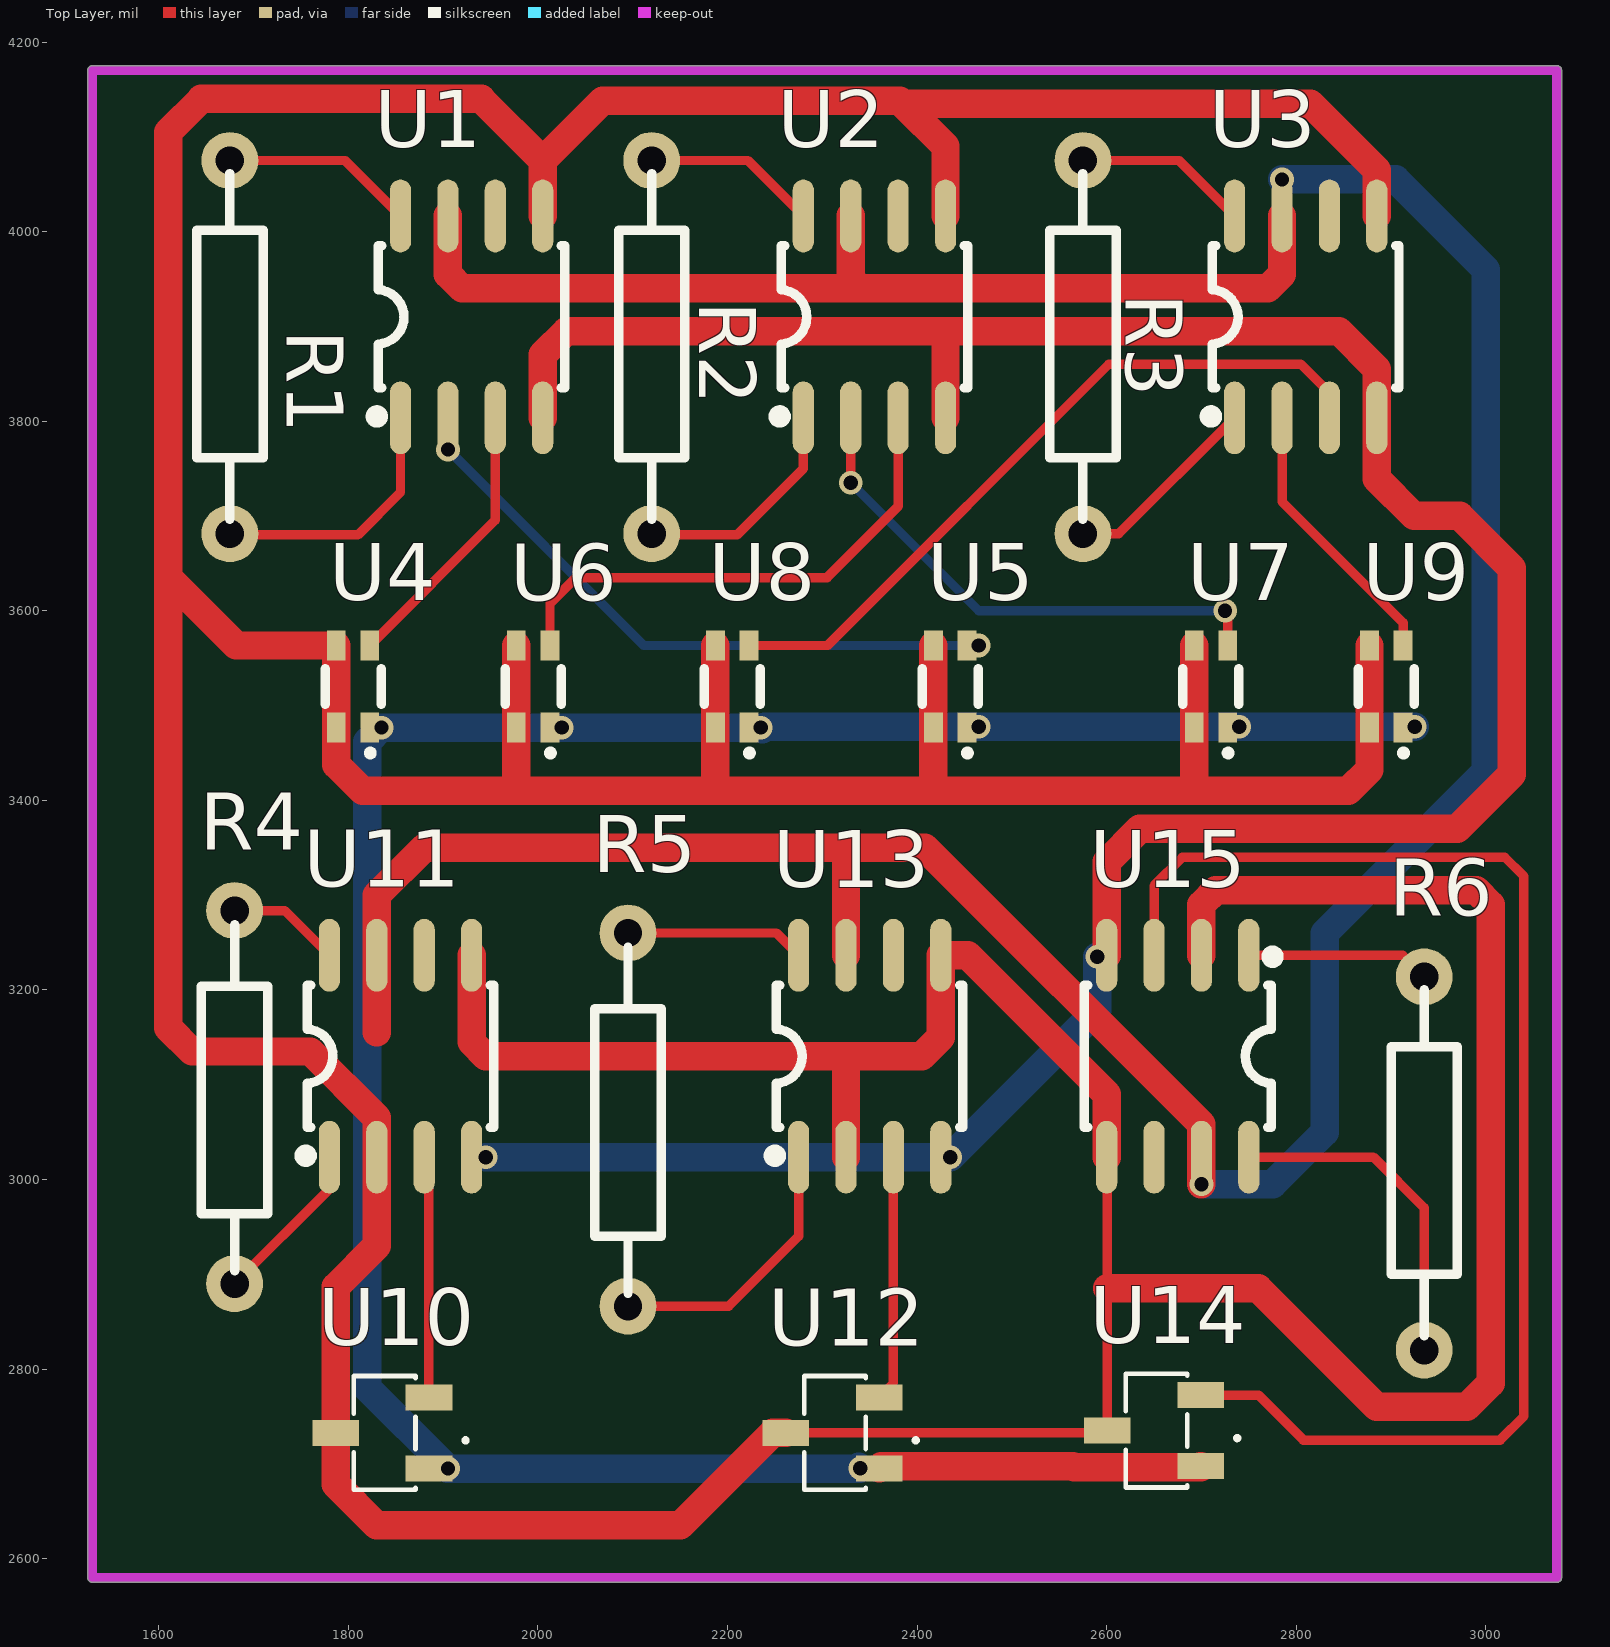
[diagram p0: Top Layer view]
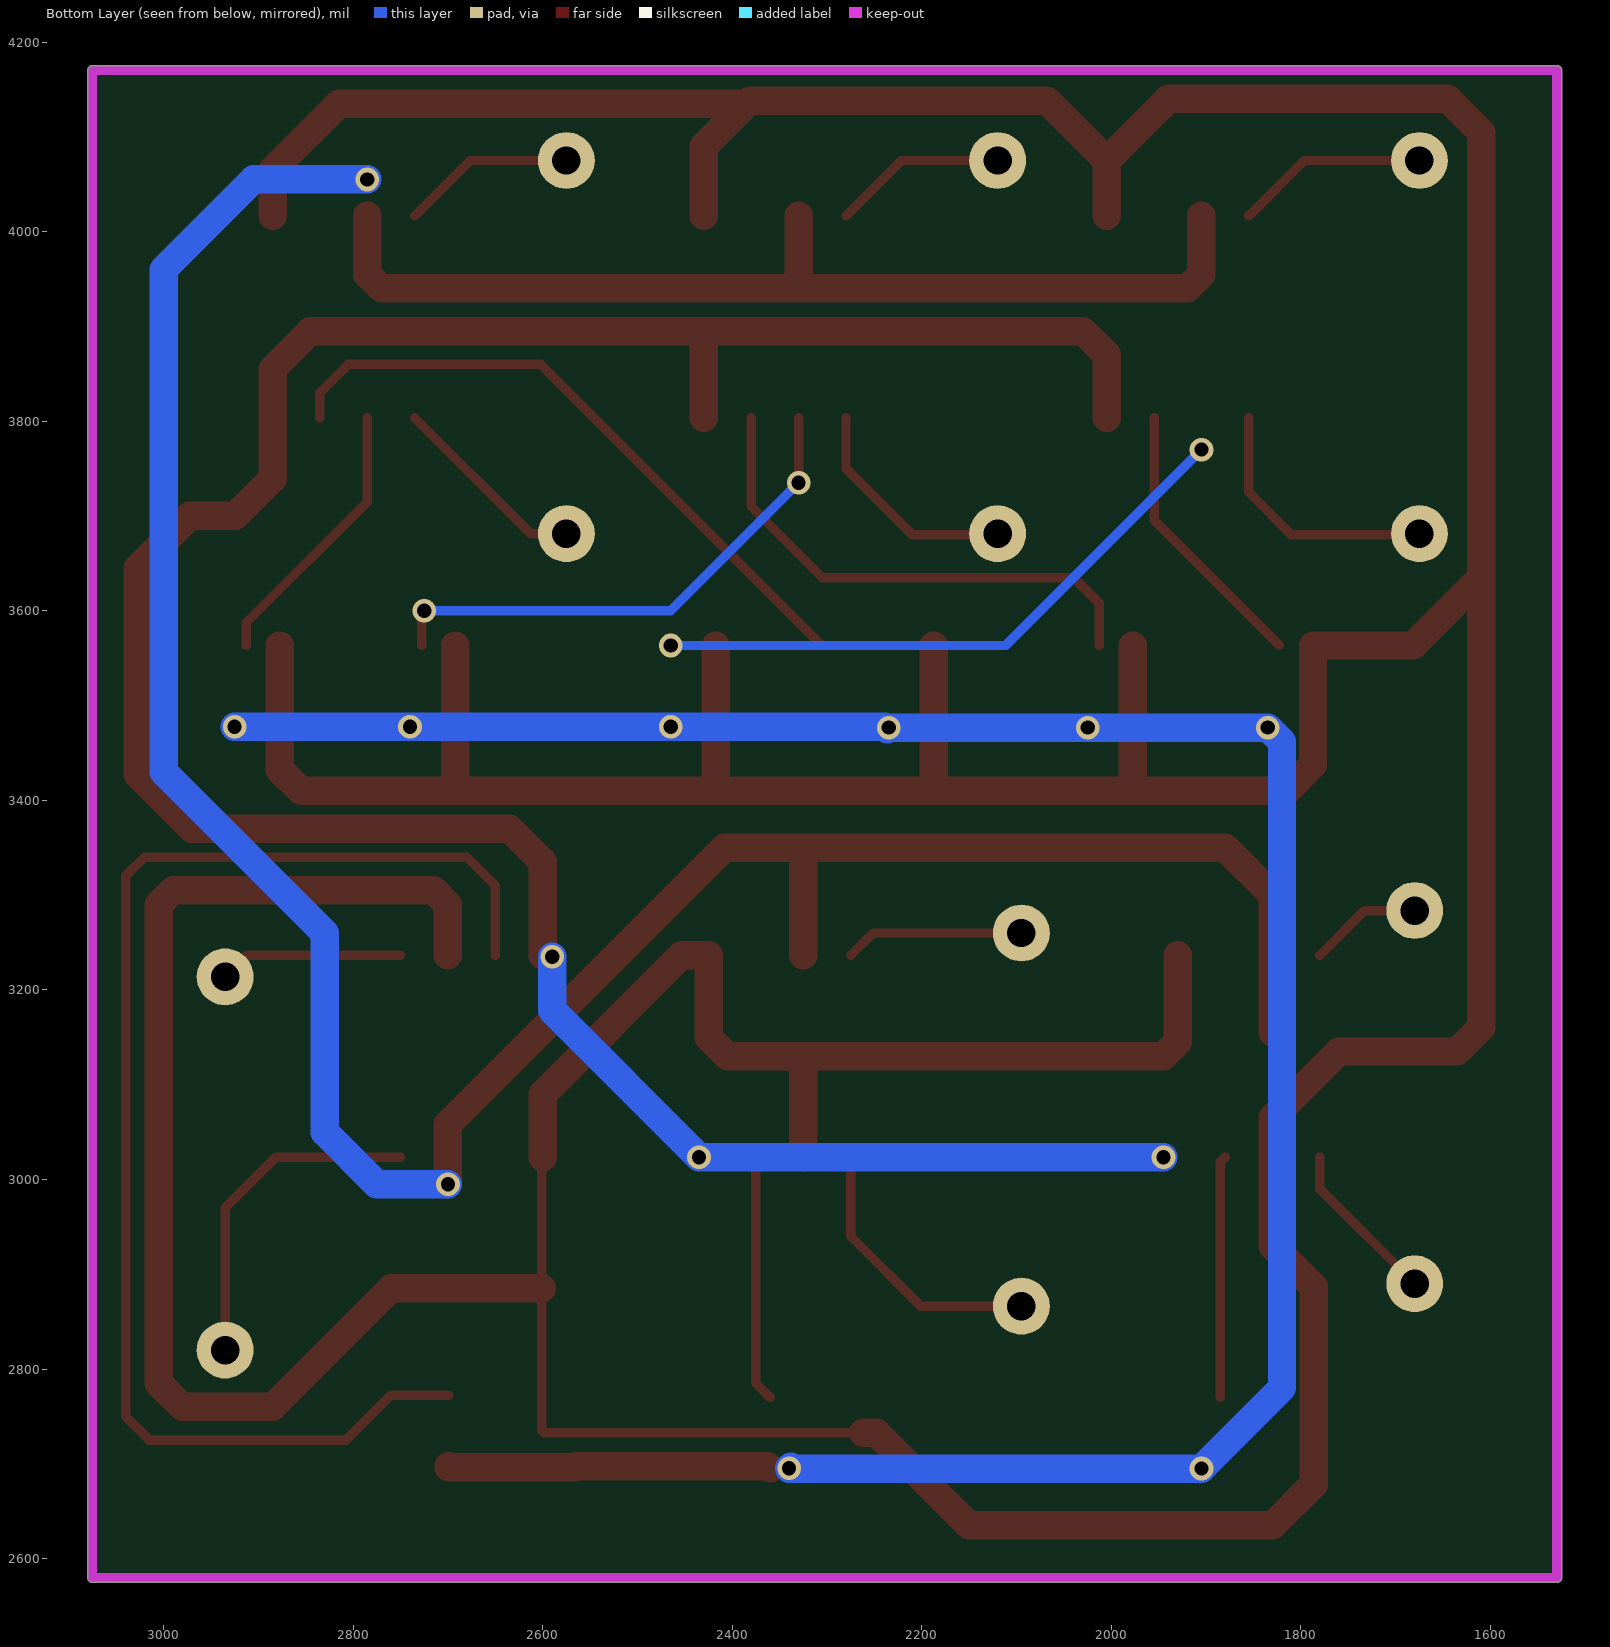
[diagram p1: Bottom Layer view, seen from below]
# Altium PCB MISC80767.PcbDoc
Units mil, origin at the board's own origin, x right, y up, seen from the top; angles counter-clockwise.
Board outline 1555.03 x 1600.03 mil, 2 copper layers (Top Layer, Bottom Layer); 21 components, 25 nets, 93 pads, 17 vias.

## Layer stack, top to bottom (the 12.6 mil dielectric is the usual default, probably not edited)
Top Solder: solder mask 0.4, Solder Resist, Dk 3.5
Top Layer: signal copper 1.4
Dielectric 1: dielectric 12.6, FR-4, Dk 4.8
Bottom Layer: signal copper 1.4
Bottom Solder: solder mask 0.4, Solder Resist, Dk 3.5

## Board outline
1530,2574.99 cw(c1530,2580) 1524.98,2580 1524.98,4170 cw(c1530,4170) 1530,4175.02 3075,4175.02 cw(c3075,4170) 3080.01,4170 3080.01,2580 cw(c3075,2580) 3075,2574.99

## Design rules (kind name [scope] priority, off if disabled: settings)
Clearance [All] p1: gap=10
PolygonConnect [All] p1: connectstyle=Relief reliefconductorwidth=10 reliefentries=4 polygonreliefangle="90 Angle" airgapwidth=10
RoutingVias [All] p1: holewidth=28 width=50 viastyle="Through Hole" minholewidth=28 minwidth=50 maxholewidth=28 maxwidth=50
SolderMaskExpansion [All] p1: expansion=4
Width [All] p1: maxlimit=222 minlimit=10 preferedwidth=10 minimp=50.000000 maximp=50.000000 favimp=50.000000
30 further rules are at their usual default settings.

## Components (designator, comment, footprint, x,y, rotation, side; value= is the part's Value field where it differs from the comment)
R1 "1K" R一般电阻/10mm 1675,3681.3 r90 top
R2 "1K" R一般电阻/10mm 2120,3681.3 r90 top
R3 "1K" R一般电阻/10mm 2575,3681.3 r90 top
R4 "5.5K" R一般电阻/10mm 1680,3283.7 r270 top
R5 "5.5K" R一般电阻/10mm 2095,3260 r270 top
R6 "5.5K" R一般电阻/10mm 2935,2820 r90 top
U1 "AD620ARZ-REEL" SOIC-8_L5.0-W4.0-P1.27-LS6.0-BL 1930,3910 r0 top
U2 "AD620ARZ-REEL" SOIC-8_L5.0-W4.0-P1.27-LS6.0-BL 2355,3910 r0 top
U3 "AD620ARZ-REEL" SOIC-8_L5.0-W4.0-P1.27-LS6.0-BL 2810,3910 r0 top
U4 "HG106A" SOP-4_L1.5-W1.5-P0.90-LS2.5-BL 1805,3520 r90 top
U5 "HG106A" SOP-4_L1.5-W1.5-P0.90-LS2.5-BL 2435,3520 r90 top
U6 "HG106A" SOP-4_L1.5-W1.5-P0.90-LS2.5-BL 1995,3520 r90 top
U7 "HG106A" SOP-4_L1.5-W1.5-P0.90-LS2.5-BL 2710,3520 r90 top
U8 "HG106A" SOP-4_L1.5-W1.5-P0.90-LS2.5-BL 2205,3520 r90 top
U9 "HG106A" SOP-4_L1.5-W1.5-P0.90-LS2.5-BL 2895,3520 r90 top
U10 "JSM3144" SOT-23-3_L2.9-W1.6-P1.90-LS2.8-BR-CW 1835.8,2732.6 r0 top
U11 "AD620ARZ-REEL" SOIC-8_L5.0-W4.0-P1.27-LS6.0-BL 1855,3130 r0 top
U12 "JSM3144" SOT-23-3_L2.9-W1.6-P1.90-LS2.8-BR-CW 2310.8,2732.6 r0 top
U13 "AD620ARZ-REEL" SOIC-8_L5.0-W4.0-P1.27-LS6.0-BL 2350,3130 r0 top
U14 "JSM3144" SOT-23-3_L2.9-W1.6-P1.90-LS2.8-BR-CW 2650,2735 r0 top
U15 "AD620ARZ-REEL" SOIC-8_L5.0-W4.0-P1.27-LS6.0-BL 2675,3130 r180 top

## Footprints (in the part's own frame and the unit in brackets; to place one, negate y for a bottom-side part, rotate by r counter-clockwise, add the part's x,y. Pads: shape width x height; smd on the part's side, far side on the other; paste and mask are expansions set on the pad)
R一般电阻/10mm [mil]
  round 60 hole 30: 1(0,0) 2(393.7,0)
  silkscreen extent 15,-35 380,35, body extent -15,-47 409,47, height 95
SOIC-8_L5.0-W4.0-P1.27-LS6.0-BL [mil]
  oval 22.38x76.78 smd: 1(-75,-106.5) 2(-25,-106.5) 3(25,-106.5) 4(75,-106.5) 5(75,106.5) 6(25,106.5) 7(-25,106.5) 8(-75,106.5)
  silkscreen extent -106,-111 98,75
SOP-4_L1.5-W1.5-P0.90-LS2.5-BL [mm]
  rect 0.8x0.5 smd paste+0 mask+0.05: 1(-1.1,-0.45) 2(1.1,-0.45) 3(1.1,0.45) 4(-1.1,0.45)
  silkscreen extent -1.82,-0.75 0.47,0.75
SOT-23-3_L2.9-W1.6-P1.90-LS2.8-BR-CW [mm]
  rect 1.25x0.7 smd: 1(1.25,-0.95) 2(-1.25,0) 3(1.25,0.95)
  silkscreen extent -0.76,-1.52 2.28,1.52

## Part data
R1 R2 R3 R4 R5 R6: library part R一般电阻
U4 U5 U6 U7 U8 U9: library part HG106A_1

## Via types
v1: diameter 25, hole 15, Top Layer to Bottom Layer, 17 vias

## Nets (pads, with @x,y where several pads share a name; then routed paths per layer and width w, separated by ;. In a path a pad name is that pad's centre, name@x,y a point inside that pad or via, vN(x,y) a via of type N, cw(c..) or ccw(c..) an arc to the next point about the centre after c; other vN are vias at no path point)
+5: U1.7 U2.7 U3.7 U11.7 U13.7 U15.7 | length 3818.9
  Top Layer w30: 1830,3155 U11.7 1830,3300 1880,3350 2320,3350 ; U1.7 1905,3955 1920,3940 2340,3940 ; U13.7 2325,3345 2320,3350 ; U2.7 2330,3950 2340,3940 ; v1(2700,2995) U15.7 2700,3058.12 2408.12,3350 2320,3350 ; U3.7 2785,3955 2770,3940 2340,3940
  Bottom Layer w30: v1(2700,2995) 2775,2995 2830,3050 2830,3260 3000,3430 3000,3960 2905,4055 v1(2785,4055)
-5: U1.4 U2.4 U3.4 U11.4 U13.4 U15.4 | length 2911.8
  Top Layer w30: U1.4 2005,3870 2030,3895 2435,3895 ; U2.4 2430,3890 2435,3895 ; U15.4 2600,3335 2635,3370 2970,3370 3027.5,3427.5 3027.5,3644.93 2972.43,3700 2924.26,3700 2885,3739.26 U3.4 2885,3855 2845,3895 2435,3895
  Bottom Layer w30: v1(1945,3023.5) v1(2435,3023.5) 2590,3178.5 v1(2590,3235)
GND: U1.5 U2.5 U3.5 U4.3 U4.4 U5.3 U5.4 U6.3 U6.4 U7.3 U7.4 U8.3 U8.4 U9.3 U9.4 U10.2 U11.2 U11.5 U12.2 U13.2 U13.5 U14.2 U15.2 U15.5 | length 9018.6
  Top Layer w10: U12.2 2598.4,2732.6 U14.2 2600.8,2885 2600.8,3022.7 U15.5
  Top Layer w30: U11.5 1930,3145 1945,3130 2325,3130 ; U6.3 U6.4 1977.28,3412.28 1975,3410 ; U1.5 2005,4075 ; U8.3 U8.4 2187.28,3412.28 2185,3410 ; U12.2 2247.6,2732.6 2150,2635 1830,2635 1786.6,2678.4 U10.2 1786.6,2886.6 1830,2930 U11.2 1830,3065 1760,3135 1635,3135 1610,3160 1610,3635 ; U13.2 2325,3130 ; U5.3 U5.4 2417.28,3412.72 2420,3410 ; U2.5 2430,4090 2385,4135 ; U15.5 2600,3090 2453.5,3236.5 U13.5 2425,3150 2405,3130 2325,3130 ; 2600.8,2885 2760,2885 2885,2760 2980,2760 3005,2785 3005,3290 2990,3305 2715,3305 2700,3290 U15.2 ; U7.3 U7.4 2692.28,3412.72 2695,3410 ; U9.3 U9.4 2877.28,3432.28 2855,3410 2695,3410 ; U3.5 2885,4065 2815,4135 2385,4135 ; 1610,3635 1610,4105 1645,4140 1940,4140 2005,4075 ; 1610,3635 1681.69,3563.31 U4.3 U4.4 1787.28,3437.72 1815,3410 1975,3410 ; 1975,3410 2185,3410 ; 2005,4075 2068.24,4138.24 2381.76,4138.24 2385,4135 ; 2185,3410 2420,3410 ; 2420,3410 2695,3410
NetR1_1: R1.1 U1.1 | length 283.4
  Top Layer w10: R1.1@1675,3695 1690,3680 1810,3680 1855,3725 U1.1
NetR1_2: R1.2 U1.8 | length 209.9
  Top Layer w10: R1.2@1675,4088.7 1688.7,4075 1796.5,4075 U1.8
NetR2_1: R2.1 U2.1 | length 248.7
  Top Layer w10: R2.1@2120,3695 2135,3680 2210,3680 2280,3750 U2.1
NetR2_2: R2.2 U2.8 | length 189.9
  Top Layer w10: R2.2@2120,4088.7 2133.7,4075 2221.5,4075 U2.8
NetR3_1: R3.1 U3.1 | length 210.6
  Top Layer w10: R3.1 2612.8,3681.3 U3.1
NetR3_2: R3.2 U3.8 | length 184.2
  Top Layer w10: R3.2 2676.5,4075 U3.8
NetR4_1: R4.1 U11.8 | length 119.6
  Top Layer w10: R4.1 1732.8,3283.7 U11.8
NetR4_2: R4.2 U11.1 | length 174.9
  Top Layer w10: R4.2 1780,2990 U11.1
NetR5_1: R5.1 U13.8 | length 189.7
  Top Layer w10: R5.1 2251.5,3260 U13.8
NetR5_2: R5.2 U13.1 | length 294
  Top Layer w10: R5.2 2201.3,2866.3 2275,2940 U13.1
NetR6_1: R6.1 U15.8 | length 357.2
  Top Layer w10: U15.8 2881.5,3023.5 2935,2970 R6.1
NetR6_2: R6.2 U15.1 | length 194.4
  Top Layer w10: U15.1 2912.2,3236.5 R6.2
NetU1_2: U1.2 U5.2 | length 645.6
  Bottom Layer w10: v1(1905,3770) 2111.69,3563.31 v1(2465,3563.31)
NetU1_3: U1.3 U4.2 | length 295
  Top Layer w10: U4.2 1955,3695.59 U1.3
NetU2_2: U2.2 U7.2 | length 557.2
  Top Layer w10: v1(2330,3735) U2.2 ; v1(2725,3600) 2727.72,3597.28 U7.2
  Bottom Layer w10: v1(2330,3735) 2465,3600 v1(2725,3600)
NetU2_3: U2.3 U6.2 | length 547.6
  Top Layer w10: U6.2 2012.72,3607.72 2040,3635 2305,3635 2380,3710 U2.3
NetU3_2: U3.2 U9.2 | length 293.1
  Top Layer w10: U3.2 2785,3715 2912.72,3587.28 U9.2
NetU3_3: U3.3 U8.2 | length 774.1
  Top Layer w10: U8.2 2305.59,3563.31 2602.28,3860 2805,3860 2835,3830 U3.3
NetU10_3: U10.3 U11.3 | length 255.6
  Top Layer w10: U11.3 1885,3018.5 U10.3
NetU12_3: U12.3 U13.3 | length 259.7
  Top Layer w10: U12.3 2375,2785 U13.3
NetU14_3: U14.3 U15.3 | length 1425
  Top Layer w10: U15.3 2650,3310 2680,3340 3020,3340 3040,3320 3040,2750 3015,2725 2807.6,2725 2760.2,2772.4 U14.3
VCC: U4.1 U5.1 U6.1 U7.1 U8.1 U9.1 U10.1 U12.1 U14.1 | length 2694.2
  Top Layer w30: U12.1 2362.4,2697.6 2564.46,2697.6 2565.84,2696.22 2699.2,2696.22 U14.1
  Bottom Layer w30: v1@2338.51,2696.69 v1(2340,2695.2) 2339.8,2695 v1(1905,2695) 1820,2780 1820,3461.69 v1(1835,3476.69) v1(2025,3476.69) v1(2235,3476.69) 2236.69,3475 2239.29,3477.6 v1(2465,3477.6) v1(2740,3477.6) v1(2925,3477.6)
pads on no net: U1.6 U2.6 U3.6 U11.6 U13.6 U15.6

## Keep-outs
Keep-Out Layer:
  lines w10: 1530,2580 3075,2580 3075,4170 1570,4170 1530,4170 1530,2580